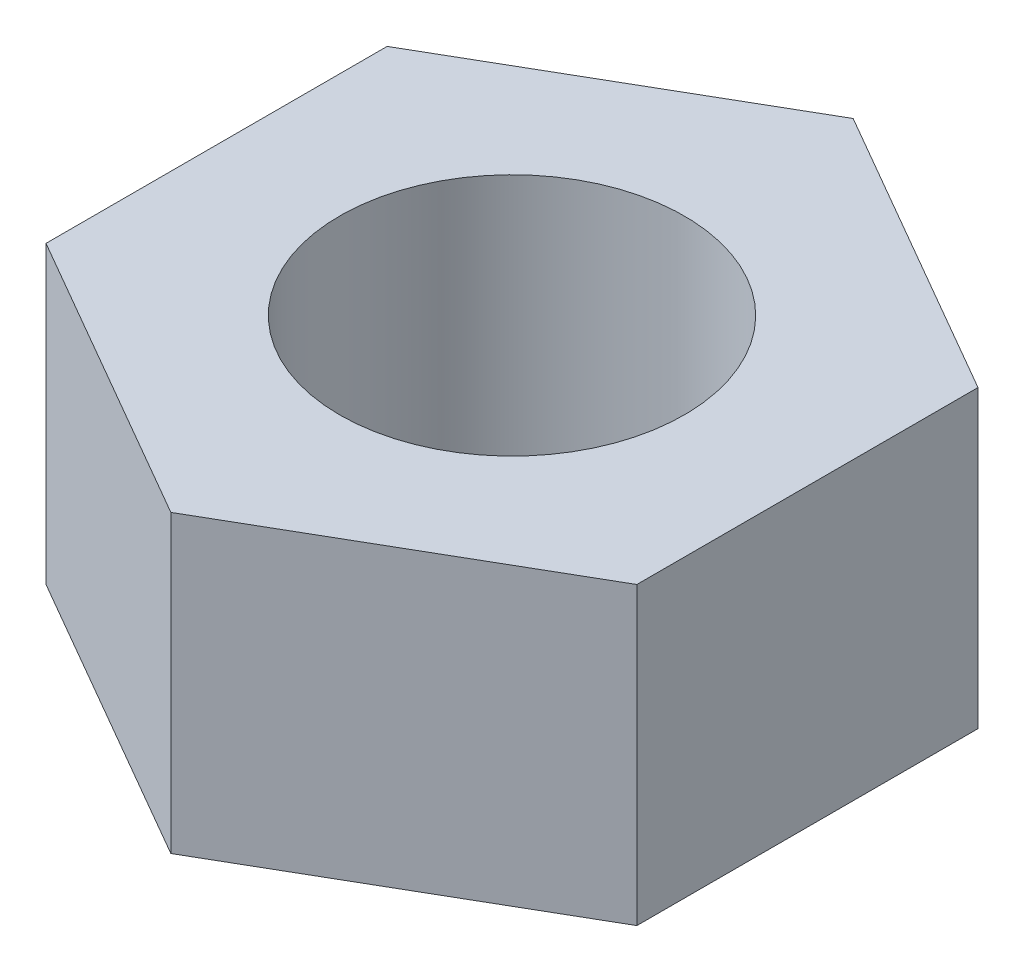
SolidWorks part; units mm, degrees
ref_plane "前视基准面" through (0, 0, 0) normal (0, 0, 1) x (1, 0, 0)
ref_plane "上视基准面" through (0, 0, 0) normal (0, 1, 0) x (1, 0, 0)
ref_plane "右视基准面" through (0, 0, 0) normal (1, 0, 0) x (0, 0, -1)
sketch "草图1" plane through (0, 0, 0) normal (0, 1, 0) x (1, 0, 0)
  line L0 (0, 0.866) -> (0, 20.5922) construction
  line L1 (0, 17.3205) -> (-15, 8.6603)
  line L2 (-15, 8.6603) -> (-15, -8.6603)
  line L3 (-15, -8.6603) -> (0, -17.3205)
  line L4 (0, -17.3205) -> (15, -8.6603)
  line L5 (15, -8.6603) -> (15, 8.6603)
  line L6 (15, 8.6603) -> (0, 17.3205)
  circle A0 centre (0, 0) radius 15 construction
  dimension "D1" = 30
extrude "凸台-拉伸1" add sketch "草图1" along normal blind 15
hole_wizard "M20 螺纹孔1" positions "草图3" profile "草图2" tap size "M20" standard "ISO" end condition through all
sketch "草图3" plane through (0, 15, 0) normal (0, 1, 0) x (1, 0, 0)
  point P0 (0, 0)
sketch "草图2" plane through (0, 15, 0) normal (1, 0, 0) x (0, 0, 1)
  line L0 (0, 0) -> (0, 15)
  line L1 (0, 15) -> (8.75, 15)
  line L2 (8.75, 15) -> (8.75, 0)
  line L5 (8.75, 0) -> (0, 0)
  line L11 (0, -6.35) -> (0, 107.95) construction
  dimension "通孔螺纹孔钻头直径" = 17.5
  dimension "通孔螺纹孔钻头深度" = 15
cosmetic thread "孔螺蚊线1"
